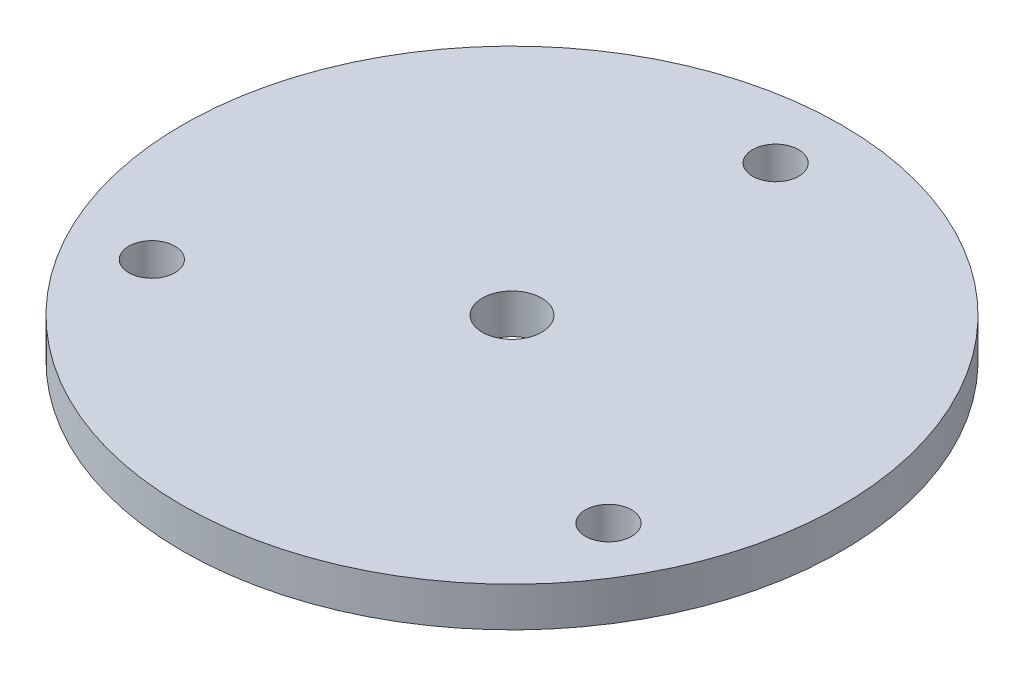
SolidWorks part; units mm, degrees
material "Q235A"
ref_plane "Front Plane" through (0, 0, 0) normal (0, 0, 1) x (1, 0, 0)
ref_plane "Top Plane" through (0, 0, 0) normal (0, 1, 0) x (1, 0, 0)
ref_plane "Right Plane" through (0, 0, 0) normal (1, 0, 0) x (0, 0, -1)
sketch "Sketch1" plane through (0, 0, 0) normal (0, 1, 0) x (1, 0, 0)
  circle A0 centre (0, 0) radius 50
  dimension "D1" = 100
extrude "Boss-Extrude1" add sketch "Sketch1" along normal mid plane 6
sketch "Sketch2" plane through (0, 3, 0) normal (0, 1, 0) x (1, 0, 0)
  line L0 (-60.6832, 0) -> (57.4974, 0) construction
  line L1 (0, 52.7944) -> (0, -54.8389) construction
  circle A2 centre (0, 40) radius 3.5
  circle A3 centre (0, 0) radius 40 construction
  circle A4 centre (34.641, -20) radius 3.5
  circle A5 centre (-34.641, -20) radius 3.5
  point P16 (0, 0)
  dimension "D1" = 80
  dimension "D2" = 7
  dimension "D3" = 3
extrude "Cut-Extrude1" cut sketch "Sketch2" against normal through all
hole_wizard "M10x1.0 Tapped Hole1" positions "Sketch4" profile "Sketch3" tap size "M10x1.0" standard "GB" end condition through all
sketch "Sketch4" plane through (0, 3, 0) normal (0, 1, 0) x (1, 0, 0)
  point P0 (0, 0)
sketch "Sketch3" plane through (0, 3, 0) normal (1, 0, 0) x (0, 0, 1)
  line L0 (0, 0) -> (0, 6)
  line L1 (0, 6) -> (4.5, 6)
  line L2 (4.5, 6) -> (4.5, 0)
  line L5 (4.5, 0) -> (0, 0)
  line L11 (0, -6.35) -> (0, 107.95) construction
  dimension "通孔螺纹孔钻头直径" = 9
  dimension "通孔螺纹孔钻头深度" = 6
cosmetic thread "Cosmetic Thread1"
